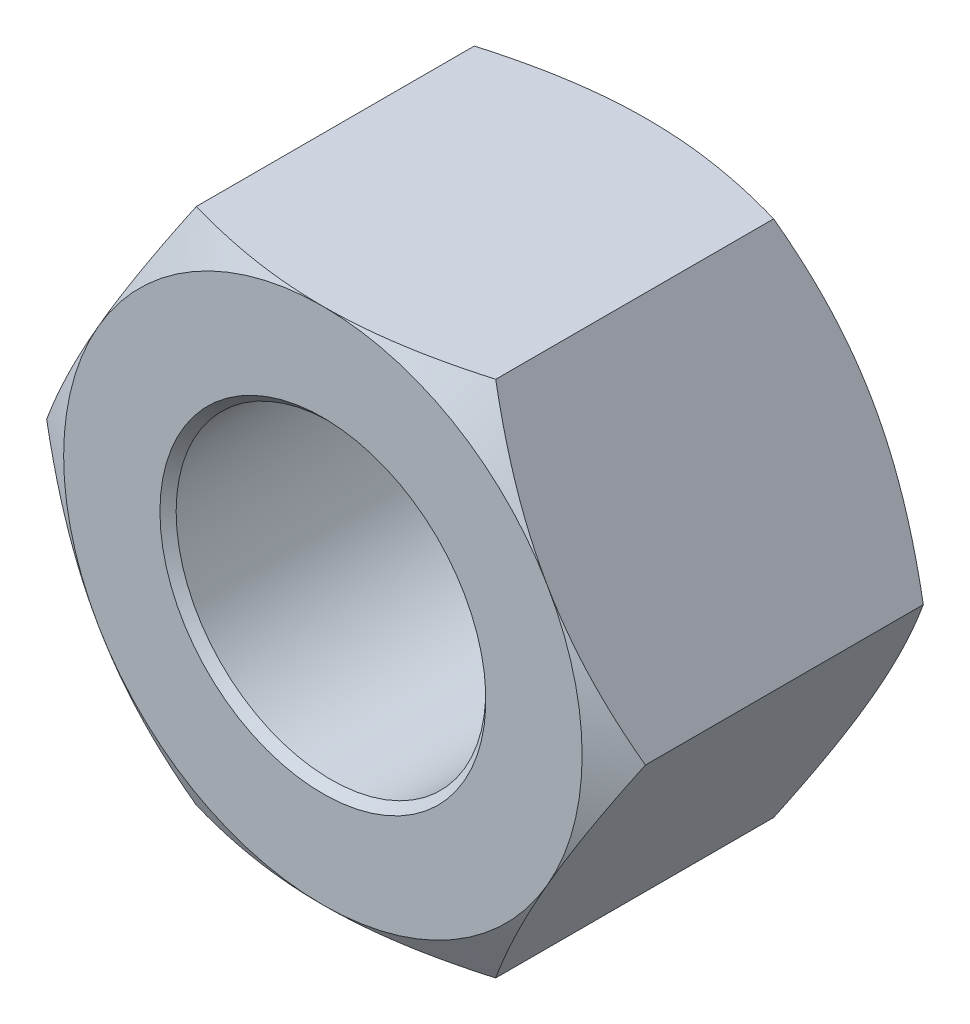
from build123d import *

# Parameters (mm, degrees)
SKETCH_1_R          = 9.646875
EXTRUDE_483_DEPTH   = 20.2
SKETCH_2_OUTSIDE_W  = 163.884
SKETCH_2_OUTSIDE_H  = 158.886
SKETCH_2_OUTSIDE_R  = 16.151373781
CUT_EXTRUDE_1_DEPTH = 32.886194113
CUT_EXTRUDE_1_DRAFT = -60
SKETCH_3_OUTSIDE_W  = 163.884
SKETCH_3_OUTSIDE_H  = 158.886
SKETCH_3_OUTSIDE_R  = 16.151373781
CUT_EXTRUDE_2_DEPTH = 32.886194113
CUT_EXTRUDE_2_DRAFT = -60
CHAMFER_1_SIZE      = 0.505


with BuildPart() as part:
    # 草图1 → Extrude 483 (new body)
    with BuildSketch(Plane.XY):
        Polygon((9.325, 16.151373781), (-9.325, 16.151373781), (-18.65, 0), (-9.325, -16.151373781), (9.325, -16.151373781), (18.65, 0), align=None)
        Circle(SKETCH_1_R, mode=Mode.SUBTRACT)
    extrude(amount=EXTRUDE_483_DEPTH)


with BuildPart() as cut_extrude_1_tool:
    # 草图2 outside → 切除-拉伸1 (with draft: the straight prism first)
    with BuildSketch(Plane(origin=(0, 0, 0), x_dir=(-1, 0, 0), z_dir=(0, 0, -1))):
        Rectangle(SKETCH_2_OUTSIDE_W, SKETCH_2_OUTSIDE_H)
        Circle(SKETCH_2_OUTSIDE_R, mode=Mode.SUBTRACT)
    extrude(amount=-CUT_EXTRUDE_1_DEPTH)
    # 切除-拉伸1: the draft: its side faces are tilted about the plane it starts from
    cut_extrude_1_sides = [cut_extrude_1_tool.faces().sort_by_distance(p)[0] for p in [
        (0, -79.443, 16.443097056),
        (-81.942, 0, 16.443097056),
        (0, 79.443, 16.443097056),
        (81.942, 0, 16.443097056),
        (16.151373781, 0, 16.443097056),
    ]]
    draft(cut_extrude_1_sides, Plane(origin=(0, 0, 0), x_dir=(-1, 0, 0), z_dir=(0, 0, -1)), CUT_EXTRUDE_1_DRAFT)


with BuildPart() as part_1:
    add(part.part)

    # 切除-拉伸1: cut by cut_extrude_1_tool
    add(cut_extrude_1_tool.part, mode=Mode.SUBTRACT)


with BuildPart() as cut_extrude_2_tool:
    # 草图3 outside → 切除-拉伸2 (with draft: the straight prism first)
    with BuildSketch(Plane.XY.offset(20.2)):
        Rectangle(SKETCH_3_OUTSIDE_W, SKETCH_3_OUTSIDE_H)
        Circle(SKETCH_3_OUTSIDE_R, mode=Mode.SUBTRACT)
    extrude(amount=-CUT_EXTRUDE_2_DEPTH)
    # 切除-拉伸2: the draft: its side faces are tilted about the plane it starts from
    cut_extrude_2_sides = [cut_extrude_2_tool.faces().sort_by_distance(p)[0] for p in [
        (0, -79.443, 3.756902944),
        (81.942, 0, 3.756902944),
        (0, 79.443, 3.756902944),
        (-81.942, 0, 3.756902944),
        (-16.151373781, 0, 3.756902944),
    ]]
    draft(cut_extrude_2_sides, Plane.XY.offset(20.2), CUT_EXTRUDE_2_DRAFT)


with BuildPart() as part_2:
    add(part_1.part)

    # 切除-拉伸2: cut by cut_extrude_2_tool
    add(cut_extrude_2_tool.part, mode=Mode.SUBTRACT)

    # 倒角1
    chamfer_1_edges = [part_2.edges().sort_by_distance(p)[0] for p in [
        (-9.646875, 0, 0),
        (-9.646875, 0, 20.2),
    ]]
    chamfer(chamfer_1_edges, length=CHAMFER_1_SIZE)


solid = part_2.part
